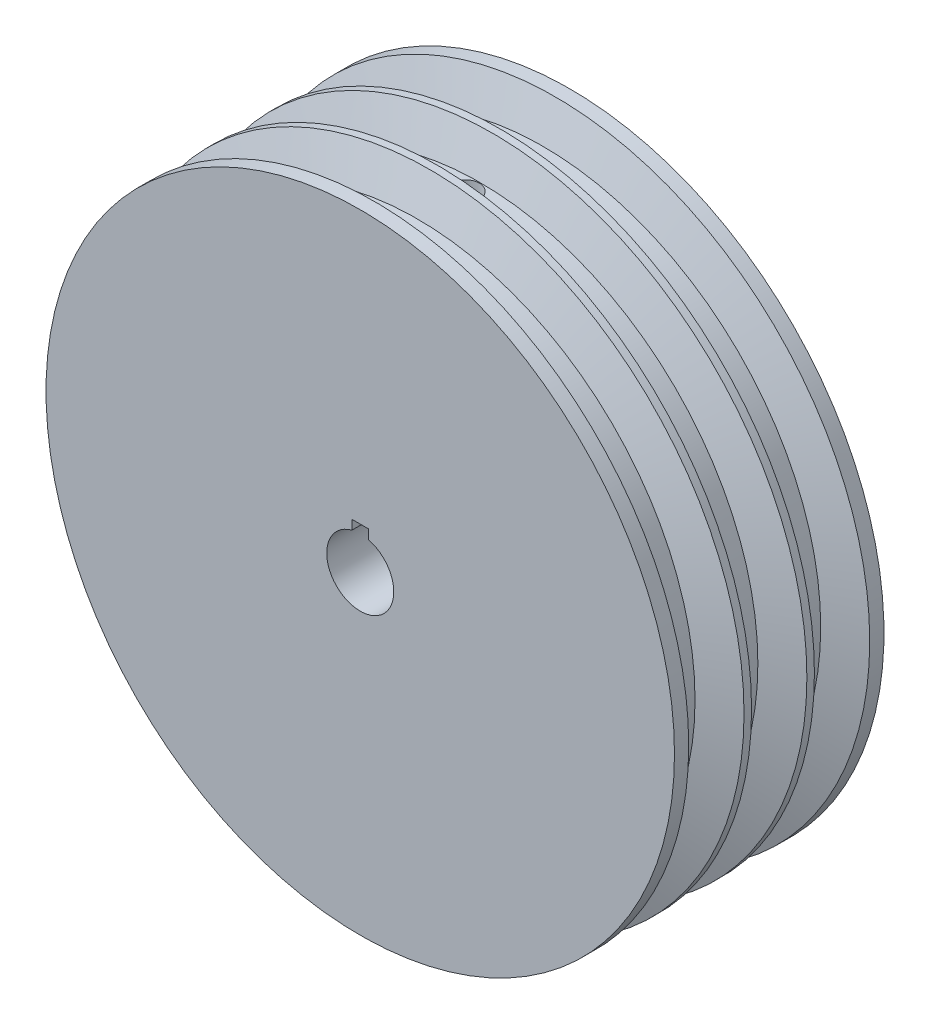
SolidWorks part; units mm, degrees
ref_plane "Front Plane" through (0, 0, 0) normal (0, 0, 1) x (1, 0, 0)
ref_plane "Top Plane" through (0, 0, 0) normal (0, 1, 0) x (1, 0, 0)
ref_plane "Right Plane" through (0, 0, 0) normal (1, 0, 0) x (0, 0, -1)
sketch "Sketch1" plane through (0, 0, 0) normal (0, 0, 1) x (1, 0, 0)
  circle A0 centre (0, 0) radius 75
  dimension "D1" = 150
extrude "Boss-Extrude1" add sketch "Sketch1" along normal mid plane 80
sketch "Sketch2" plane through (0, 0, 40) normal (0, 0, 1) x (1, 0, 0)
  circle A0 centre (0, 0) radius 8
  dimension "D1" = 16
extrude "Cut-Extrude1" cut sketch "Sketch2" against normal blind 150
sketch "Sketch4" plane through (0, 0, 0) normal (1, 0, 0) x (0, 0, -1)
  line L0 (-40, 75) -> (-40, -75) construction
  line L1 (-40, 75) -> (-40, -75) construction
  line L2 (-40, 75) -> (-40, -75) construction
  line L3 (-40, 75) -> (-36.6, 75)
  line L4 (-36.6, 75) -> (-33.6043, 66.3)
  line L5 (-21.6, 75) -> (-18.6043, 66.3)
  line L6 (-30, 66.3) -> (-30, 134.1405) construction
  line L7 (-33.6043, 66.3) -> (-26.3957, 66.3)
  line L8 (-23.4, 75) -> (-26.3957, 66.3)
  line L15 (-23.4, 75) -> (-21.6, 75)
  line L19 (10, 161.0505) -> (-40, 161.0505)
  line L20 (-40, 161.0505) -> (-40, 75)
  line L21 (0, 0) -> (121.1492, 0) construction
  line L22 (-18.6043, 66.3) -> (-11.3957, 66.3)
  line L23 (-8.4, 75) -> (-11.3957, 66.3)
  line L24 (-8.4, 75) -> (-6.6, 75)
  line L25 (-6.6, 75) -> (-3.6043, 66.3)
  line L26 (-3.6043, 66.3) -> (3.6043, 66.3)
  line L27 (6.6, 75) -> (3.6043, 66.3)
  line L32 (0, 66.3) -> (0, 132.7741) construction
  line L36 (6.6, 75) -> (10, 75)
  line L39 (21.6, 75) -> (23.4, 75) [skipped]
  line L40 (38.6, 75) -> (90.6382, 75) [skipped]
  line L41 (11.3957, 66.3) -> (18.6043, 66.3) [skipped]
  line L42 (21.6, 75) -> (18.6043, 66.3) [skipped]
  line L43 (23.4, 75) -> (26.3957, 66.3) [skipped]
  line L44 (26.3957, 66.3) -> (33.6043, 66.3) [skipped]
  line L45 (36.6, 75) -> (33.6043, 66.3) [skipped]
  line L46 (8.4, 75) -> (11.3957, 66.3) [skipped]
  line L47 (6.6, 75) -> (8.4, 75) [skipped]
  line L48 (40, 75) -> (-40, 75) construction
  line L49 (10, 75) -> (10, 161.0505)
  dimension "D1" = 10
  dimension "D2" = 8.7
  dimension "D3" = 6.6
  dimension "D4" = 19
  dimension "D5" = 5
  dimension "D6" = 10
revolve "Cut-Revolve1" cut sketch "Sketch4" angle 360 about L21
sketch "Sketch10" plane through (0, 0, -40) normal (0, 0, -1) x (-1, 0, 0)
  circle A4 centre (0, 0) radius 100
  dimension "D1" = 200
extrude "Cut-Extrude5" cut sketch "Sketch10" against normal blind 20
sketch "Sketch11" plane through (0, 0, -20) normal (0, 0, -1) x (-1, 0, 0)
  circle A0 centre (0, 0) radius 30
  circle A3 centre (0, 0) radius 8
  circle A4 centre (0, 0) radius 8
  dimension "D2" = 60
  dimension "D1" = 0
extrude "Boss-Extrude2" add sketch "Sketch11" along normal blind 20
sketch "Sketch12" plane through (0, 0, -40) normal (0, 0, -1) x (-1, 0, 0)
  circle A2 centre (0, 0) radius 130
  circle A3 centre (0, 0) radius 130
  dimension "D1" = 100
extrude "Cut-Extrude6" cut sketch "Sketch12" against normal blind 30
sketch "Sketch13" plane through (0, 0, -10) normal (0, 0, -1) x (-1, 0, 0)
  line L1 (-2, 10) -> (2, 10)
  line L2 (-2, 10) -> (-2, 6)
  line L3 (-2, 6) -> (2, 6)
  line L4 (2, 10) -> (2, 6)
  line L5 (-2, 10) -> (2, 6) construction
  line L6 (-2, 6) -> (2, 10) construction
  circle A0 centre (0, 0) radius 8 construction
  point P0 (0, 8)
  dimension "D1" = 4
  dimension "D2" = 4
extrude "Cut-Extrude7" cut sketch "Sketch13" against normal blind 500
hole_wizard "M8 Tapped Hole1" positions "Sketch14" profile "Sketch15" tap size "M8" standard "GB"
sketch "Sketch14" plane through (0, 10, 0) normal (0, -1, 0) x (-1, 0, 0)
  point P0 (0, -15)
sketch "Sketch15" plane through (0, 10, 15) normal (1, 0, 0) x (0, 0, -1)
  line L0 (0, 0) -> (0, 65)
  line L1 (0, 65) -> (3.4, 65)
  line L2 (3.4, 65) -> (3.4, 0)
  line L5 (3.4, 0) -> (0, 0)
  line L11 (0, -6.35) -> (0, 107.95) construction
  dimension "通孔螺纹孔钻头直径" = 6.8
  dimension "通孔螺纹孔钻头深度" = 65
cosmetic thread "Hole thread 1" parameters "D2"=8
